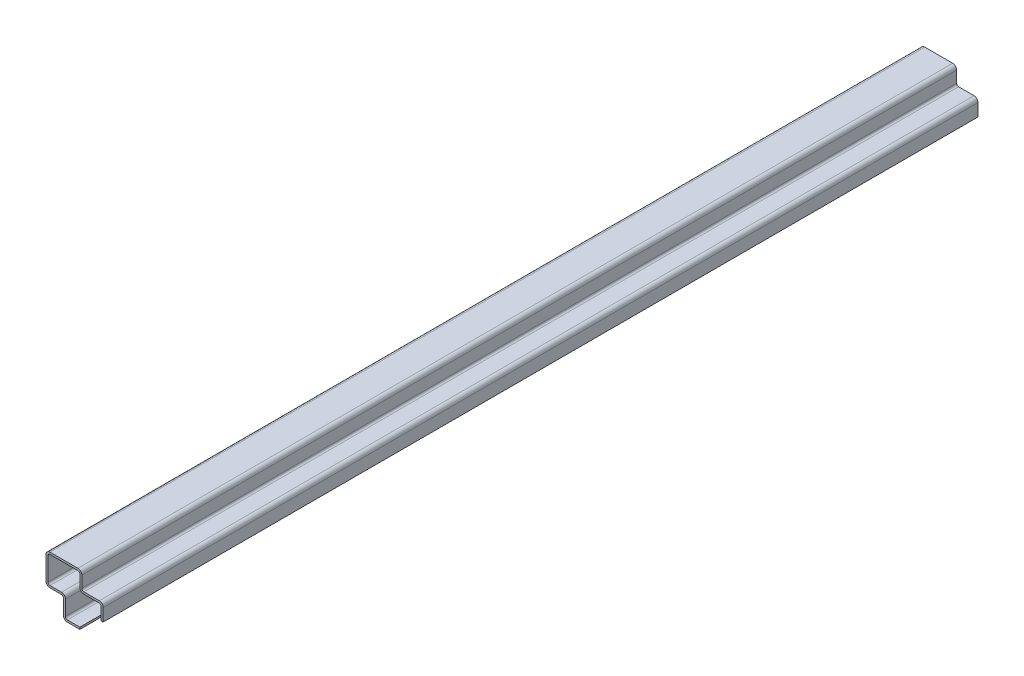
SolidWorks part; units mm, degrees
ref_plane "Front Plane" through (0, 0, 0) normal (0, 0, 1) x (1, 0, 0)
ref_plane "Top Plane" through (0, 0, 0) normal (0, 1, 0) x (1, 0, 0)
ref_plane "Right Plane" through (0, 0, 0) normal (1, 0, 0) x (0, 0, -1)
other "Configuration Table"
sketch "Sketch1" plane through (0, 0, 0) normal (0, 0, 1) x (1, 0, 0)
  line L0 (0, 0) -> (0, 38)
  line L1 (-12, 50) -> (-59, 50)
  line L2 (-65, 56) -> (-65, 91)
  line L3 (-77, 103) -> (-162, 103)
  line L4 (-174, 91) -> (-174, 21)
  line L5 (-162, 9) -> (-127, 9)
  line L6 (-121, 3) -> (-121, -43)
  line L7 (-109, -55) -> (-71, -55)
  line L8 (-71, -55) -> (-71, -49)
  line L9 (-71, -49) -> (-109, -49)
  line L10 (-115, -43) -> (-115, 3)
  line L11 (-127, 15) -> (-162, 15)
  line L12 (-168, 21) -> (-168, 91)
  line L13 (-162, 97) -> (-77, 97)
  line L14 (-71, 91) -> (-71, 56)
  line L15 (-59, 44) -> (-12, 44)
  line L16 (-6, 38) -> (-6, 0)
  line L17 (-6, 0) -> (0, 0)
  arc A0 (0, 38) -> (-12, 50) centre (-12, 38) ccw
  arc A1 (-65, 56) -> (-59, 50) centre (-59, 56) ccw
  arc A2 (-65, 91) -> (-77, 103) centre (-77, 91) ccw
  arc A3 (-162, 103) -> (-174, 91) centre (-162, 91) ccw
  arc A4 (-174, 21) -> (-162, 9) centre (-162, 21) ccw
  arc A5 (-121, 3) -> (-127, 9) centre (-127, 3) ccw
  arc A6 (-121, -43) -> (-109, -55) centre (-109, -43) ccw
  arc A7 (-115, -43) -> (-109, -49) centre (-109, -43) ccw
  arc A8 (-115, 3) -> (-127, 15) centre (-127, 3) ccw
  arc A9 (-168, 21) -> (-162, 15) centre (-162, 21) ccw
  arc A10 (-162, 97) -> (-168, 91) centre (-162, 91) ccw
  arc A11 (-71, 91) -> (-77, 97) centre (-77, 91) ccw
  arc A12 (-71, 56) -> (-59, 44) centre (-59, 56) ccw
  arc A13 (-6, 38) -> (-12, 44) centre (-12, 38) ccw
  dimension "D1" = 12
  dimension "D2" = 6
  dimension "D3" = 65
  dimension "D4" = 115
  dimension "D5" = 168
  dimension "D6" = 9
  dimension "D7" = 49
extrude "Boss-Extrude1" add sketch "Sketch1" along normal blind 2660
